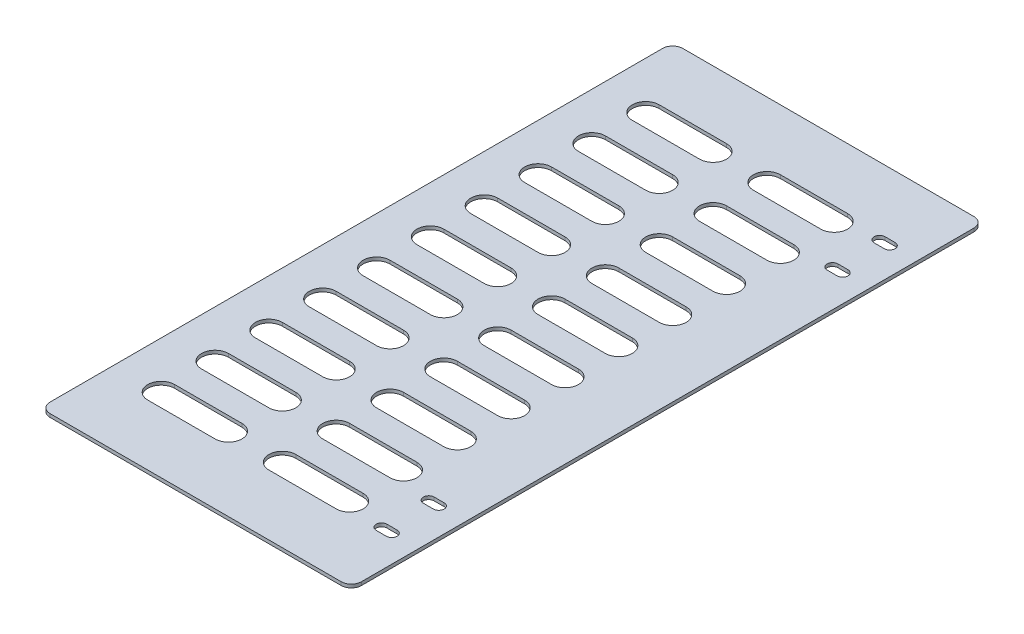
from build123d import *

# Parameters (mm, degrees)
SKETCH_1_W          = 92.5
SKETCH_1_H          = 188
EXTRUDE_1_DEPTH     = 1
FILLET_1_R          = 3
CUT_EXTRUDE_2_DEPTH = 10
CUT_EXTRUDE_3_DEPTH = 10


with BuildPart() as part:
    # 草图1 → 凸台-拉伸1 (new body)
    with BuildSketch(Plane(origin=(0, 0, 0), x_dir=(1, 0, 0), z_dir=(0, 1, 0))):
        Rectangle(SKETCH_1_W, SKETCH_1_H)
    extrude(amount=EXTRUDE_1_DEPTH)

    # 圆角1
    fillet_1_edges = [part.edges().sort_by_distance(p)[0] for p in [
        (46.25, 0.5, 94),
        (-46.25, 0.5, 94),
        (-46.25, 0.5, -94),
        (46.25, 0.5, -94),
    ]]
    fillet(fillet_1_edges, radius=FILLET_1_R)

    # 草图3 → 切除-拉伸2 (cut)
    with BuildSketch(Plane(origin=(0, 1, 0), x_dir=(1, 0, 0), z_dir=(0, 1, 0))):
        with BuildLine():
            Line((35.25, 61.6), (38.25, 61.6))
            ThreePointArc((38.25, 61.6), (39.85, 60), (38.25, 58.4))
            Line((38.25, 58.4), (35.25, 58.4))
            ThreePointArc((35.25, 58.4), (33.65, 60), (35.25, 61.6))
        make_face()
        with BuildLine():
            Line((35.25, 75.6), (38.25, 75.6))
            ThreePointArc((38.25, 75.6), (39.85, 74), (38.25, 72.4))
            Line((38.25, 72.4), (35.25, 72.4))
            ThreePointArc((35.25, 72.4), (33.65, 74), (35.25, 75.6))
        make_face()
        with BuildLine():
            Line((35.25, -61.6), (38.25, -61.6))
            ThreePointArc((38.25, -61.6), (39.85, -60), (38.25, -58.4))
            Line((38.25, -58.4), (35.25, -58.4))
            ThreePointArc((35.25, -58.4), (33.65, -60), (35.25, -61.6))
        make_face()
        with BuildLine():
            Line((35.25, -75.6), (38.25, -75.6))
            ThreePointArc((38.25, -75.6), (39.85, -74), (38.25, -72.4))
            Line((38.25, -72.4), (35.25, -72.4))
            ThreePointArc((35.25, -72.4), (33.65, -74), (35.25, -75.6))
        make_face()
    extrude(amount=-CUT_EXTRUDE_2_DEPTH, mode=Mode.SUBTRACT)

    # 草图4 → 切除-拉伸3 (cut)
    with BuildSketch(Plane(origin=(0, 1, 0), x_dir=(1, 0, 0), z_dir=(0, 1, 0))):
        with BuildLine():
            Line((-32.25, 12), (-12.25, 12))
            ThreePointArc((-12.25, 12), (-8.25, 8), (-12.25, 4))
            Line((-12.25, 4), (-32.25, 4))
            ThreePointArc((-32.25, 4), (-36.25, 8), (-32.25, 12))
        make_face()
        with BuildLine():
            Line((3.75, 12), (23.75, 12))
            ThreePointArc((23.75, 12), (27.75, 8), (23.75, 4))
            Line((23.75, 4), (3.75, 4))
            ThreePointArc((3.75, 4), (-0.25, 8), (3.75, 12))
        make_face()
        with BuildLine():
            Line((-32.25, 28), (-12.25, 28))
            ThreePointArc((-12.25, 28), (-8.25, 24), (-12.25, 20))
            Line((-12.25, 20), (-32.25, 20))
            ThreePointArc((-32.25, 20), (-36.25, 24), (-32.25, 28))
        make_face()
        with BuildLine():
            Line((3.75, 28), (23.75, 28))
            ThreePointArc((23.75, 28), (27.75, 24), (23.75, 20))
            Line((23.75, 20), (3.75, 20))
            ThreePointArc((3.75, 20), (-0.25, 24), (3.75, 28))
        make_face()
        with BuildLine():
            Line((-32.25, 44), (-12.25, 44))
            ThreePointArc((-12.25, 44), (-8.25, 40), (-12.25, 36))
            Line((-12.25, 36), (-32.25, 36))
            ThreePointArc((-32.25, 36), (-36.25, 40), (-32.25, 44))
        make_face()
        with BuildLine():
            Line((3.75, 44), (23.75, 44))
            ThreePointArc((23.75, 44), (27.75, 40), (23.75, 36))
            Line((23.75, 36), (3.75, 36))
            ThreePointArc((3.75, 36), (-0.25, 40), (3.75, 44))
        make_face()
        with BuildLine():
            Line((-32.25, 60), (-12.25, 60))
            ThreePointArc((-12.25, 60), (-8.25, 56), (-12.25, 52))
            Line((-12.25, 52), (-32.25, 52))
            ThreePointArc((-32.25, 52), (-36.25, 56), (-32.25, 60))
        make_face()
        with BuildLine():
            Line((3.75, 60), (23.75, 60))
            ThreePointArc((23.75, 60), (27.75, 56), (23.75, 52))
            Line((23.75, 52), (3.75, 52))
            ThreePointArc((3.75, 52), (-0.25, 56), (3.75, 60))
        make_face()
        with BuildLine():
            Line((-32.25, 76), (-12.25, 76))
            ThreePointArc((-12.25, 76), (-8.25, 72), (-12.25, 68))
            Line((-12.25, 68), (-32.25, 68))
            ThreePointArc((-32.25, 68), (-36.25, 72), (-32.25, 76))
        make_face()
        with BuildLine():
            Line((3.75, 76), (23.75, 76))
            ThreePointArc((23.75, 76), (27.75, 72), (23.75, 68))
            Line((23.75, 68), (3.75, 68))
            ThreePointArc((3.75, 68), (-0.25, 72), (3.75, 76))
        make_face()
        with BuildLine():
            Line((3.75, -76), (23.75, -76))
            ThreePointArc((23.75, -76), (27.75, -72), (23.75, -68))
            Line((23.75, -68), (3.75, -68))
            ThreePointArc((3.75, -68), (-0.25, -72), (3.75, -76))
        make_face()
        with BuildLine():
            Line((-32.25, -76), (-12.25, -76))
            ThreePointArc((-12.25, -76), (-8.25, -72), (-12.25, -68))
            Line((-12.25, -68), (-32.25, -68))
            ThreePointArc((-32.25, -68), (-36.25, -72), (-32.25, -76))
        make_face()
        with BuildLine():
            Line((3.75, -60), (23.75, -60))
            ThreePointArc((23.75, -60), (27.75, -56), (23.75, -52))
            Line((23.75, -52), (3.75, -52))
            ThreePointArc((3.75, -52), (-0.25, -56), (3.75, -60))
        make_face()
        with BuildLine():
            Line((-32.25, -60), (-12.25, -60))
            ThreePointArc((-12.25, -60), (-8.25, -56), (-12.25, -52))
            Line((-12.25, -52), (-32.25, -52))
            ThreePointArc((-32.25, -52), (-36.25, -56), (-32.25, -60))
        make_face()
        with BuildLine():
            Line((3.75, -44), (23.75, -44))
            ThreePointArc((23.75, -44), (27.75, -40), (23.75, -36))
            Line((23.75, -36), (3.75, -36))
            ThreePointArc((3.75, -36), (-0.25, -40), (3.75, -44))
        make_face()
        with BuildLine():
            Line((-32.25, -44), (-12.25, -44))
            ThreePointArc((-12.25, -44), (-8.25, -40), (-12.25, -36))
            Line((-12.25, -36), (-32.25, -36))
            ThreePointArc((-32.25, -36), (-36.25, -40), (-32.25, -44))
        make_face()
        with BuildLine():
            Line((3.75, -28), (23.75, -28))
            ThreePointArc((23.75, -28), (27.75, -24), (23.75, -20))
            Line((23.75, -20), (3.75, -20))
            ThreePointArc((3.75, -20), (-0.25, -24), (3.75, -28))
        make_face()
        with BuildLine():
            Line((-32.25, -28), (-12.25, -28))
            ThreePointArc((-12.25, -28), (-8.25, -24), (-12.25, -20))
            Line((-12.25, -20), (-32.25, -20))
            ThreePointArc((-32.25, -20), (-36.25, -24), (-32.25, -28))
        make_face()
        with BuildLine():
            Line((3.75, -12), (23.75, -12))
            ThreePointArc((23.75, -12), (27.75, -8), (23.75, -4))
            Line((23.75, -4), (3.75, -4))
            ThreePointArc((3.75, -4), (-0.25, -8), (3.75, -12))
        make_face()
        with BuildLine():
            Line((-32.25, -12), (-12.25, -12))
            ThreePointArc((-12.25, -12), (-8.25, -8), (-12.25, -4))
            Line((-12.25, -4), (-32.25, -4))
            ThreePointArc((-32.25, -4), (-36.25, -8), (-32.25, -12))
        make_face()
    extrude(amount=-CUT_EXTRUDE_3_DEPTH, mode=Mode.SUBTRACT)


solid = part.part
